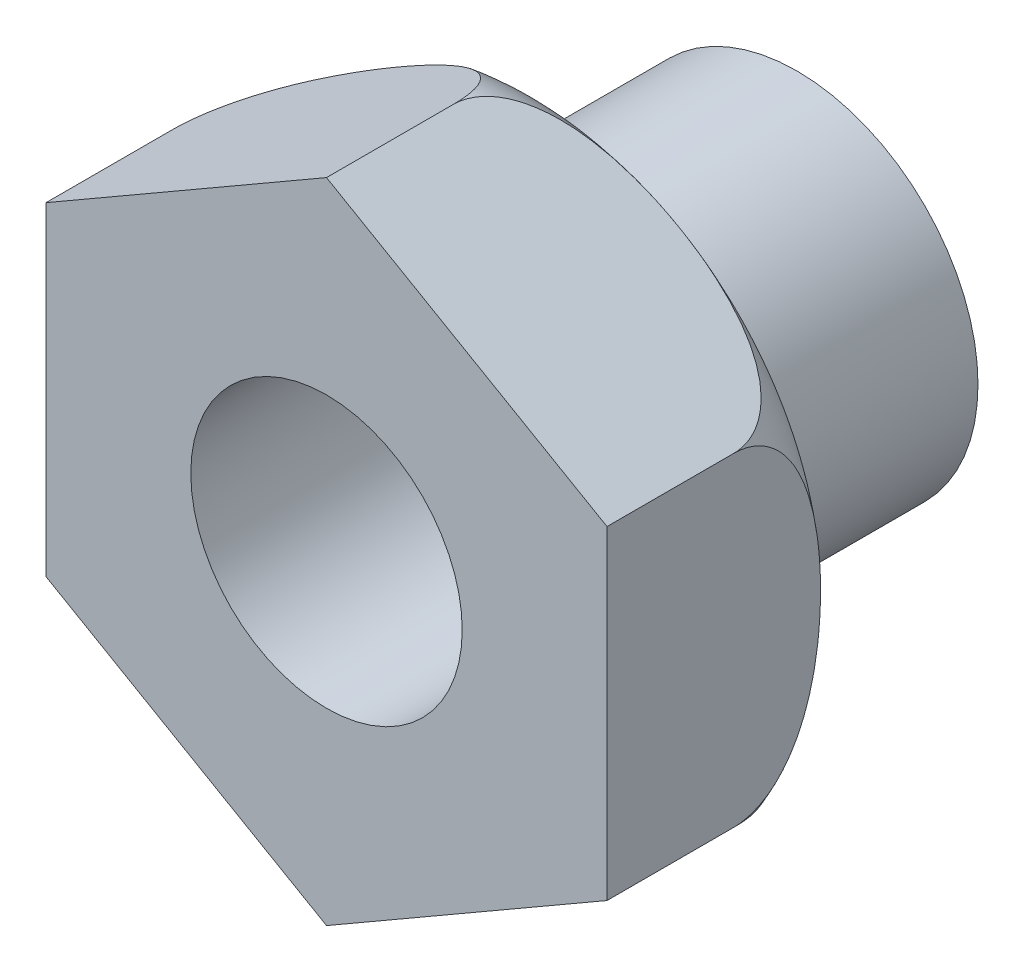
SolidWorks part; units mm, degrees
ref_plane "Front Plane" through (0, 0, 0) normal (0, 0, 1) x (1, 0, 0)
ref_plane "Top Plane" through (0, 0, 0) normal (0, 1, 0) x (1, 0, 0)
ref_plane "Right Plane" through (0, 0, 0) normal (1, 0, 0) x (0, 0, -1)
sketch "Sketch1" plane through (0, 0, 0) normal (0, 0, 1) x (1, 0, 0)
  line L1 (77.5, 44.7446) -> (0, 89.4893)
  line L2 (0, 89.4893) -> (-77.5, 44.7446)
  line L3 (-77.5, 44.7446) -> (-77.5, -44.7446)
  line L4 (-77.5, -44.7446) -> (0, -89.4893)
  line L5 (0, -89.4893) -> (77.5, -44.7446)
  line L6 (77.5, -44.7446) -> (77.5, 44.7446)
  circle A0 centre (0, 0) radius 77.5 construction
  dimension "D1" = 155
extrude "Boss-Extrude1" add sketch "Sketch1" along normal blind 65
sketch "Sketch2" plane through (0, 0, 0) normal (1, 0, 0) x (0, 0, -1)
  line L0 (-65, 89.4893) -> (0, 89.4893) construction
  line L1 (0, 44.7446) -> (0, 89.4893) construction
  line L2 (0, 59.4893) -> (0, 89.4893)
  line L3 (0, 89.4893) -> (-30, 89.4893)
  line L4 (-90.104, 0) -> (40.6351, 0) construction
  arc A0 (-30, 89.4893) -> (0, 59.4893) centre (-30, 59.4893) cw
  dimension "D1" = 30
revolve "Cut-Revolve1" cut sketch "Sketch2" angle 360 about L4
sketch "Sketch3" plane through (0, 0, 0) normal (0, 0, -1) x (-1, 0, 0)
  circle A0 centre (0, 0) radius 50
  circle A1 centre (0, 0) radius 37.5
  dimension "D1" = 100
  dimension "D2" = 75
extrude "Boss-Extrude2" add sketch "Sketch3" along normal blind 65
sketch "Sketch4" plane through (0, 0, 65) normal (0, 0, 1) x (1, 0, 0)
  circle A0 centre (0, 0) radius 37.5
  dimension "D1" = 75
extrude "Cut-Extrude2" cut sketch "Sketch4" against normal up to surface (130 mm away) up to face at (-50, 0, -65)
